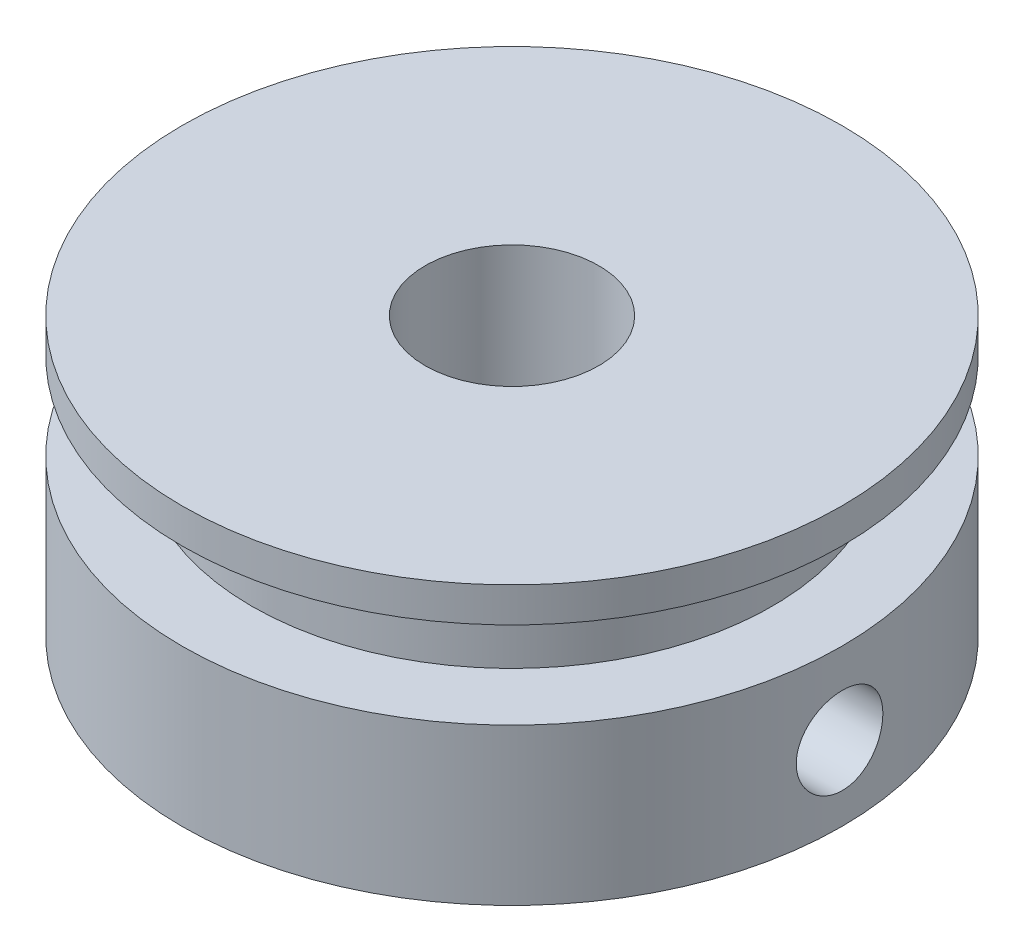
SolidWorks part; units mm, degrees
ref_plane "前视基准面" through (0, 0, 0) normal (0, 0, 1) x (1, 0, 0)
ref_plane "上视基准面" through (0, 0, 0) normal (0, 1, 0) x (1, 0, 0)
ref_plane "右视基准面" through (0, 0, 0) normal (1, 0, 0) x (0, 0, -1)
sketch "草图1" plane through (0, 0, 0) normal (0, 0, 1) x (1, 0, 0)
  line L0 (0, 34.0719) -> (0, -45.6485) construction
  line L1 (2.5, 4) -> (2.5, -4)
  line L2 (2.5, 4) -> (9.5, 4)
  line L3 (9.5, 4) -> (9.5, 3)
  line L4 (9.5, 3) -> (7.5, 3)
  line L5 (7.5, 3) -> (7.5, 0.5)
  line L6 (7.5, 0.5) -> (9.5, 0.5)
  line L7 (9.5, 0.5) -> (9.5, -4)
  line L12 (9.5, -4) -> (2.5, -4)
  point P5 (2.5, 0)
  dimension "D1" = 7
  dimension "D2" = 2.5
  dimension "D3" = 1
  dimension "D4" = 2
  dimension "D5" = 4.5
  dimension "D6" = 7
  dimension "D7" = 8
revolve "旋转1" add sketch "草图1" angle 360 about L0
ref_plane "基准面4" through (0, 0, 7.5) normal (0, 0, 1) x (1, 0, 0)
hole_wizard "M3 螺纹孔1" positions "3D草图1" profile "草图2" tap size "M3" standard "Iso"
sketch3d "3D草图1"
  point P0 (9.5, -1.8573, -0.0206)
sketch "草图2" plane through (9.5, -1.8573, -0.0206) normal (0, 1, 0) x (-0.0022, 0, -1)
  line L0 (0, 0) -> (0, 7)
  line L1 (0, 7) -> (1.25, 7)
  line L2 (1.25, 7) -> (1.25, 0)
  line L5 (1.25, 0) -> (0, 0)
  line L11 (0, -6.35) -> (0, 107.95) construction
  dimension "通孔螺纹孔钻头直径" = 2.5
  dimension "通孔螺纹孔钻头深度" = 7
cosmetic thread "孔螺蚊线1" parameters "D2"=3
